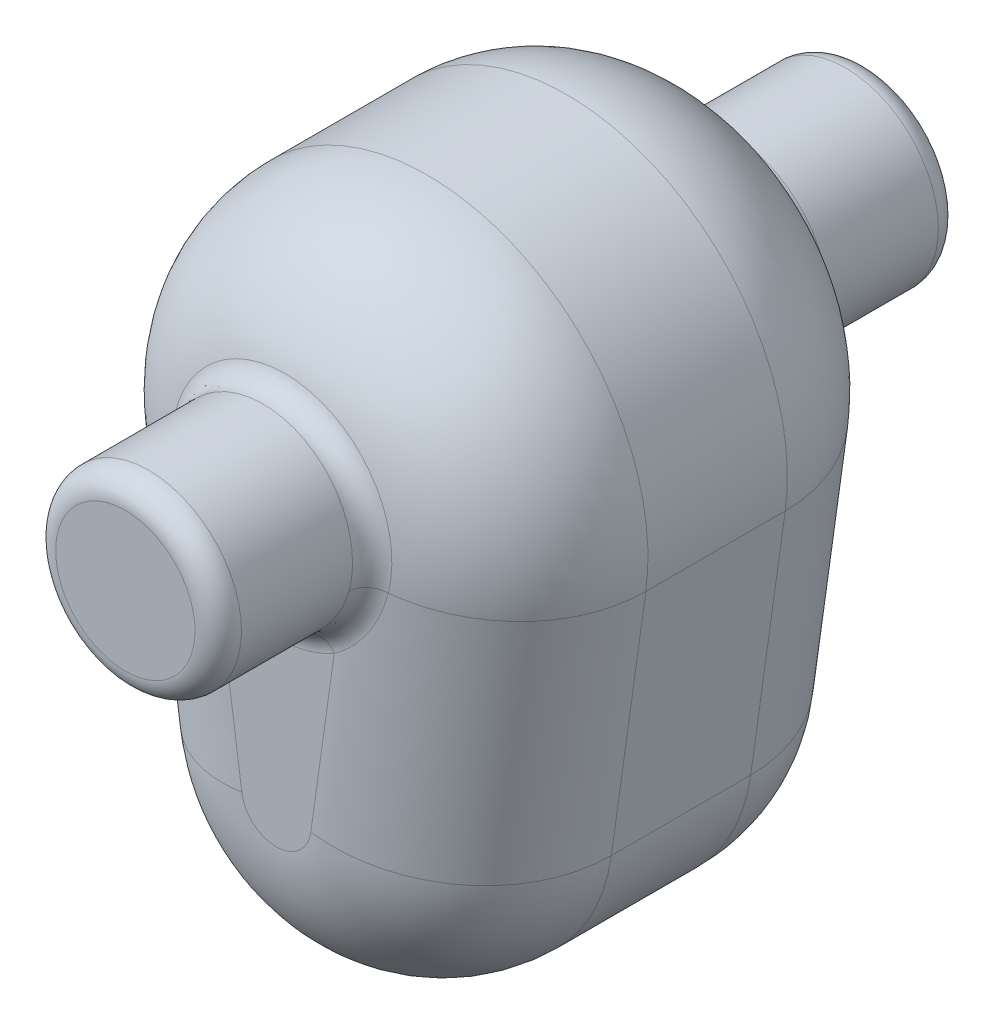
SolidWorks part; units mm, degrees
material "AISI 1045 钢，冷拔"
ref_plane "Front Plane" through (0, 0, 0) normal (0, 0, 1) x (1, 0, 0)
ref_plane "Top Plane" through (0, 0, 0) normal (0, 1, 0) x (1, 0, 0)
ref_plane "Right Plane" through (0, 0, 0) normal (1, 0, 0) x (0, 0, -1)
sketch "Sketch1" plane through (0, 0, 0) normal (0, 0, 1) x (1, 0, 0)
  line L0 (-15.0144, -2.2685) -> (-13.529, -12.8602)
  line L1 (-5.6065, -0.9491) -> (-5.6065, -3.7491) construction
  line L2 (3.8014, -2.2685) -> (2.316, -12.8602)
  line L3 (-5.6065, -10.4491) -> (-5.6065, -11.7491) construction
  arc A1 (-13.529, -12.8602) -> (2.316, -12.8602) centre (-5.6065, -11.7491) ccw
  arc A2 (3.8014, -2.2685) -> (-15.0144, -2.2685) centre (-5.6065, -0.9491) ccw
  dimension "D2" = 16
  dimension "D3" = 10.8
extrude "Boss-Extrude1" add sketch "Sketch1" along normal blind 19
fillet "Fillet1" radius 6.5 8 edges at (-5.6065, 8.5509, 0) (3.0587, -7.5643, 0) (-5.6065, -19.7491, 0) (-5.6065, -19.7491, 19) (-14.2717, -7.5643, 19) (-14.2717, -7.5643, 0) (-5.6065, 8.5509, 19) (3.0587, -7.5643, 19)
ref_plane "Plane1" through (0, 0, 9.5) normal (0, 0, 1) x (1, 0, 0)
sketch "Sketch2" plane through (0, 0, 9.5) normal (0, 0, 1) x (1, 0, 0)
  line L0 (-5.6065, 8.5509) -> (-5.6065, -21.0878) construction
  arc A0 (3.8014, -2.2685) -> (-15.0144, -2.2685) centre (-5.6065, -0.9491) ccw construction
  circle A1 centre (-5.6065, -0.4491) radius 4
  dimension "D1" = 0.5
extrude "Boss-Extrude2" add sketch "Sketch2" along normal mid plane 32
fillet "Fillet2" radius 1 2 edges at (-1.6065, -0.4491, 25.5) (-1.6065, -0.4491, -6.5)
fillet "Fillet4" radius 1 8 edges at (-5.6065, -4.4491, 19) (-2.3052, -2.7077, 18.9797) (-5.6811, 3.5503, 18.8246) (-2.0939, -2.3626, 0.0351) (-5.6065, -4.4491, 0) (-8.9078, -2.7077, 0.0203) (-9.1191, -2.3626, 18.9649) (-5.5319, 3.5503, 0.1754)
